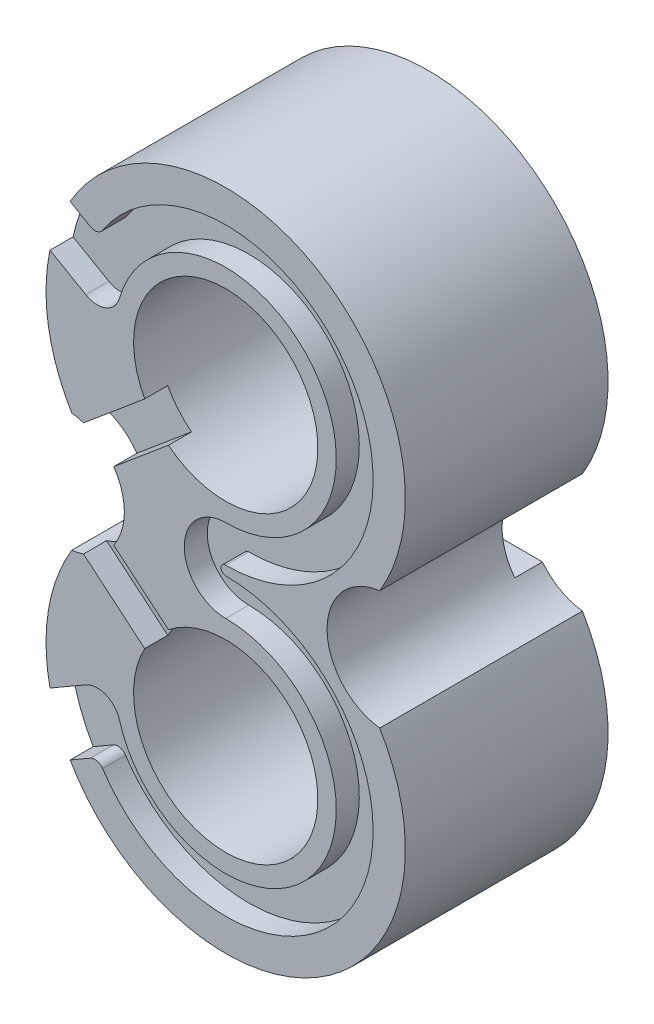
SolidWorks part; units mm, degrees
ref_plane "Front Plane" through (0, 0, 0) normal (0, 0, 1) x (1, 0, 0)
ref_plane "Top Plane" through (0, 0, 0) normal (0, 1, 0) x (1, 0, 0)
ref_plane "Right Plane" through (0, 0, 0) normal (1, 0, 0) x (0, 0, -1)
sketch "Sketch1" plane through (0, 0, 0) normal (0, 0, 1) x (1, 0, 0)
  line L1 (0, 0) -> (117.7661, 0) construction
  line L2 (0, 0) -> (0, 16.5) construction
  circle A0 centre (0, 16.5) radius 19.5
  circle A1 centre (17.5, 0) radius 6.5
  circle A2 centre (0, -16.5) radius 19.5
  circle A3 centre (0, 16.5) radius 10
  circle A4 centre (0, -16.5) radius 10
  circle A5 centre (-17.5, 0) radius 6.5
  dimension "D1" = 39
  dimension "D2" = 33
  dimension "D3" = 13
  dimension "D4" = 22
  dimension "D5" = 20
extrude "Boss-Extrude1" add sketch "Sketch1" along normal mid plane 22 contours A0 A5 A2 A1 A3 | A2 A5 A1 A0 A4 | A2 A0 | A0 A2 A1 | A0 A5 A2
sketch "Sketch2" plane through (0, 0, 11) normal (0, 0, 1) x (1, 0, 0)
  line L0 (-19.0682, 20.5808) -> (-15.1861, 18.3395)
  line L1 (-15.1861, -18.3395) -> (-19.0682, -20.5808)
  line L2 (-16.8875, -26.25) -> (-14.6969, -24.9853)
  line L3 (-14.6969, 24.9853) -> (-16.8875, 26.25)
  arc A0 (-16.8875, 26.25) -> (-19.0682, 20.5808) centre (0, 16.5) ccw
  arc A1 (-15.1861, 18.3395) -> (-11.5333, 19.8141) centre (-13.9361, 20.5045) ccw
  arc A2 (0, 4.5) -> (-11.5333, 19.8141) centre (0, 16.5) ccw
  arc A3 (0, 4.5) -> (0, -4.5) centre (0, 0) ccw
  arc A4 (-11.5333, -19.8141) -> (0, -4.5) centre (0, -16.5) ccw
  arc A5 (-11.5333, -19.8141) -> (-15.1861, -18.3395) centre (-13.9361, -20.5045) ccw
  arc A6 (-19.0682, -20.5808) -> (-16.8875, -26.25) centre (0, -16.5) ccw
  arc A7 (-13.3618, -25.3012) -> (-14.6969, -24.9853) centre (-14.1969, -25.8513) ccw
  arc A8 (-13.3618, -25.3012) -> (0, -0.5) centre (0, -16.5) ccw
  arc A9 (0, 0.5) -> (0, -0.5) centre (0, 0) ccw
  arc A10 (0, 0.5) -> (-13.3618, 25.3012) centre (0, 16.5) ccw
  arc A11 (-14.6969, 24.9853) -> (-13.3618, 25.3012) centre (-14.1969, 25.8513) ccw
extrude "Cut-Extrude1" cut sketch "Sketch2" against normal blind 2.5
sketch "Sketch3" plane through (0, 0, 11) normal (0, 0, 1) x (1, 0, 0)
  line L0 (-17.1734, 0.521) -> (1.2856, -14.9679)
  line L1 (-17.1734, 0.521) -> (-19.7446, -2.5431)
  line L2 (1.2856, -14.9679) -> (-1.2856, -18.0321)
  line L3 (-19.7446, -2.5431) -> (-1.2856, -18.0321)
  line L4 (0, -16.5) -> (-18.459, -1.011) construction
  line L5 (-7.9439, -7.2234) -> (-10.5151, -10.2876) construction
  line L6 (0, 0) -> (0, -16.5) construction
  point P1 (-9.2295, -8.7555)
  point P2 (0, -16.5)
  dimension "D1" = 50
  dimension "D2" = 4
extrude "Cut-Extrude2" cut sketch "Sketch3" against normal blind 2.5
mirror "Mirror1" about plane through (0, 0, 0) normal (0, 1, 0) of "Cut-Extrude2"
sketch "Sketch4" plane through (0, 0, -11) normal (0, 0, -1) x (-1, 0, 0)
  line L0 (12.1, 0) -> (-12.1, 0) construction
  line L1 (18.9496, -4) -> (3.5, -4)
  line L2 (18.9496, -4) -> (18.9496, 4)
  line L3 (18.9496, 4) -> (3.5, 4)
  line L4 (3.5, -4) -> (3.5, 4)
  line L5 (11.2248, 4) -> (11.2248, -4) construction
  line L6 (18.9496, 0) -> (3.5, 0) construction
  line L7 (0, 0) -> (0, -4) construction
  line L8 (0, 12.1) -> (0, -12.1) construction
  line L9 (-18.9496, 0) -> (-3.5, 0) construction
  line L10 (-11.2248, 4) -> (-11.2248, -4) construction
  line L11 (-3.5, -4) -> (-3.5, 4)
  line L12 (-18.9496, 4) -> (-3.5, 4)
  line L13 (-18.9496, -4) -> (-18.9496, 4)
  line L14 (-18.9496, -4) -> (-3.5, -4)
  point P0 (11.2248, 0)
  point P21 (-11.2248, 0)
  dimension "D1" = 8
  dimension "D2" = 7
extrude "Cut-Extrude3" cut sketch "Sketch4" against normal blind 3
fillet "Fillet1" radius 1 4 edges at (3.5, -4, -9.5) (3.5, 4, -9.5) (-3.5, -4, -9.5) (-3.5, 4, -9.5)
sketch "Sketch5" plane through (0, 0, -11) normal (0, 0, -1) x (-1, 0, 0)
  line L0 (0, 0) -> (23.6592, 0) construction
  line L1 (23.6592, 0) -> (7.3974, 9.7711)
  line L2 (23.6592, 0) -> (7.3974, -9.7711)
  line L3 (0, 6.5) -> (0, -6.5) construction
  line L4 (0, 12.1) -> (0, -12.1) construction
  line L5 (3.5, 7.1325) -> (3.5, -7.1325)
  line L6 (3.5, 6.5) -> (3.5, -6.5) construction
  circle A0 centre (0, 16.5) radius 10 construction
  arc A1 (3.5, 7.1325) -> (-9.4142, 19.8725) centre (0, 16.5) ccw
  circle A2 centre (0, -16.5) radius 10 construction
  arc A3 (7.3974, -9.7711) -> (3.5, -7.1325) centre (0, -16.5) ccw
  circle M1 centre (0, 16.5) radius 10
  arc M3 (3.5, 3) -> (4.5, 4) centre (4.5, 3) cw
  line M4 (4.5, 4) -> (12.3765, 4)
  arc M5 (12.3765, 4) -> (16.7119, 6.4521) centre (17.5, 0) cw
  arc M15 (16.7119, -6.4521) -> (12.3765, -4) centre (17.5, 0) cw
  line M16 (12.3765, -4) -> (4.5, -4)
  arc M17 (4.5, -4) -> (3.5, -3) centre (4.5, -3) cw
  circle M18 centre (0, -16.5) radius 10
  dimension "D1" = 62
  dimension "D2" = 3.5
extrude "Cut-Extrude5" cut sketch "Sketch5" against normal blind 1.5 contours L5 L1 M1 M3 M4 M5 | L5 L2 M17 M18 M15 M16
